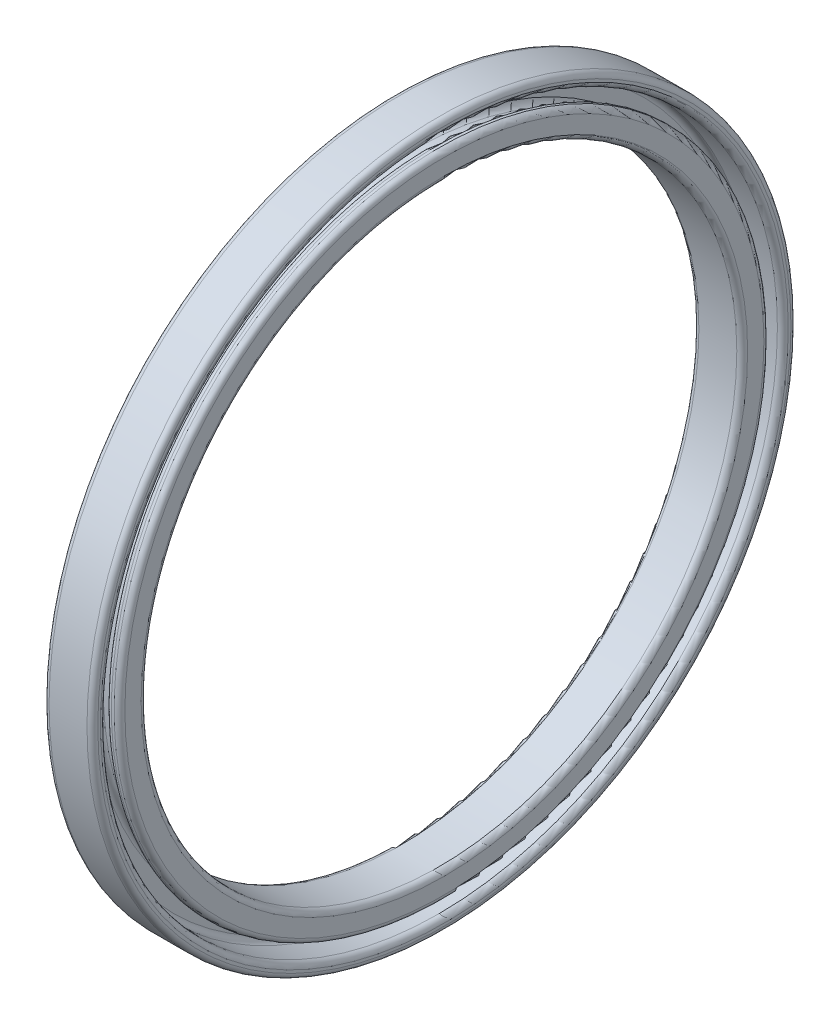
SolidWorks part; units mm, degrees
material "橡胶"
ref_plane "Front Plane" through (0, 0, 0) normal (0, 0, 1) x (1, 0, 0)
ref_plane "Top Plane" through (0, 0, 0) normal (0, 1, 0) x (1, 0, 0)
ref_plane "Right Plane" through (0, 0, 0) normal (1, 0, 0) x (0, 0, -1)
sketch "Sketch1" plane through (0, 0, 0) normal (0, 0, 1) x (1, 0, 0)
  line L0 (119.3081, 0) -> (-90.3762, 0) construction
  line L1 (2, 110) -> (16, 110)
  line L2 (18, 112) -> (18, 118)
  line L3 (16, 120) -> (15, 120)
  line L5 (7, 125) -> (16, 125)
  line L6 (18, 128) -> (18, 127)
  line L7 (16, 130) -> (2, 130)
  line L8 (0, 128) -> (0, 112)
  line L10 (11, 115) -> (7, 115)
  line L11 (5, 117) -> (5, 123)
  line L13 (13, 117) -> (13, 118)
  arc A0 (7, 115) -> (5, 117) centre (7, 117) cw
  arc A1 (5, 123) -> (7, 125) centre (7, 123) cw
  arc A2 (16, 125) -> (18, 127) centre (16, 127) ccw
  arc A3 (18, 112) -> (16, 110) centre (16, 112) cw
  arc A4 (2, 110) -> (0, 112) centre (2, 112) cw
  arc A5 (0, 128) -> (2, 130) centre (2, 128) cw
  arc A6 (18, 128) -> (16, 130) centre (16, 128) ccw
  arc A7 (18, 118) -> (16, 120) centre (16, 118) ccw
  arc A8 (15, 120) -> (13, 118) centre (15, 118) ccw
  arc A9 (13, 117) -> (11, 115) centre (11, 117) cw
  dimension "D3" = 13
  dimension "D1" = 2
  dimension "D2" = 5
  dimension "D4" = 18
  dimension "D5" = 110
  dimension "D6" = 115
revolve "Revolve1" add sketch "Sketch1" angle 360 about L0
